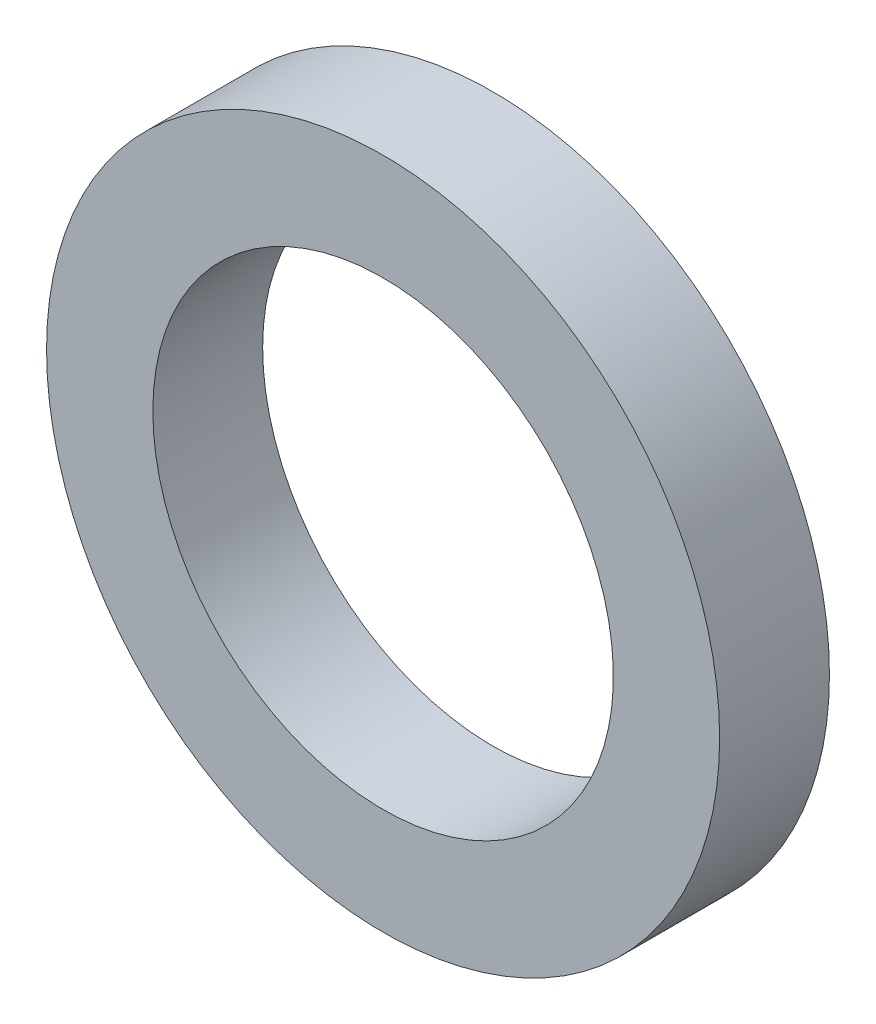
SolidWorks part; units mm, degrees
ref_plane "Front Plane" through (0, 0, 0) normal (0, 0, 1) x (1, 0, 0)
ref_plane "Top Plane" through (0, 0, 0) normal (0, 1, 0) x (1, 0, 0)
ref_plane "Right Plane" through (0, 0, 0) normal (1, 0, 0) x (0, 0, -1)
sketch "Sketch1" plane through (0, 0, 0) normal (0, 0, 1) x (1, 0, 0)
  circle A0 centre (0, 0) radius 9.5
  circle A1 centre (0, 0) radius 6.5
  dimension "D1" = 19
  dimension "D2" = 13
extrude "Boss-Extrude1" add sketch "Sketch1" along normal blind 3.1
